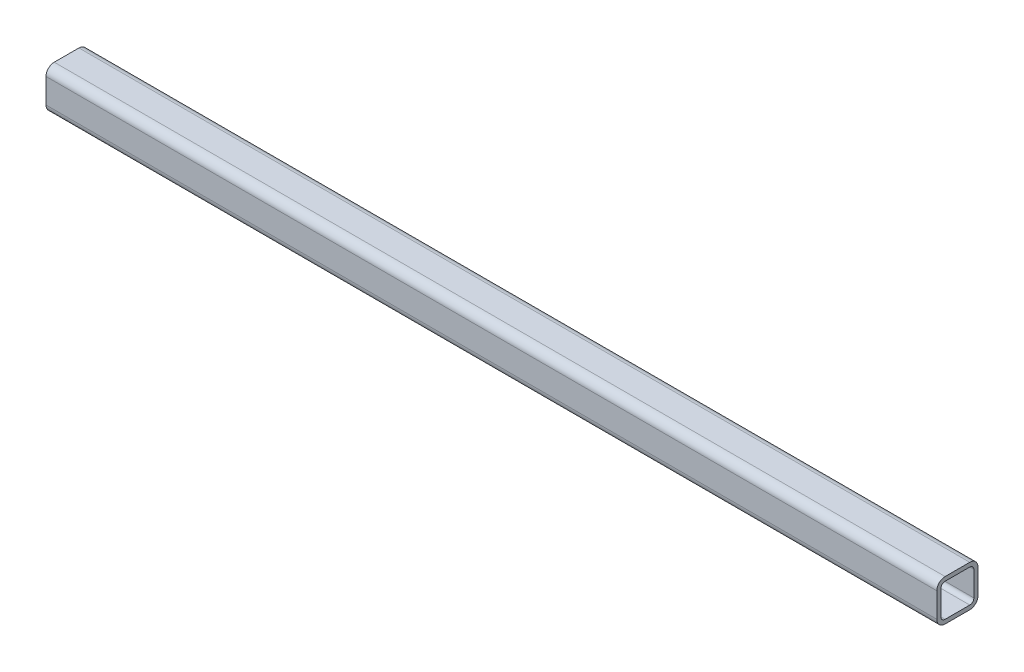
from build123d import *

# Parameters (mm, degrees)
GB_6728_1986_040_X_40_X_4_1_DEPTH = 866


with BuildPart() as part:
    # Sketch1 → Gb／6728-1986方形空心型钢 040 X 40 X 4(1) (new body)
    with BuildSketch(Plane(origin=(-433, 0, 0), x_dir=(0, 0, -1), z_dir=(1, 0, 0))):
        with BuildLine():
            Line((-12, -20), (12, -20))
            ThreePointArc((12, -20), (17.656854249, -17.656854249), (20, -12))
            Line((20, -12), (20, 12))
            ThreePointArc((20, 12), (17.656854249, 17.656854249), (12, 20))
            Line((12, 20), (-12, 20))
            ThreePointArc((-12, 20), (-17.656854249, 17.656854249), (-20, 12))
            Line((-20, 12), (-20, -12))
            ThreePointArc((-20, -12), (-17.656854249, -17.656854249), (-12, -20))
        make_face()
        with BuildLine():
            Line((-12, -16), (12, -16))
            ThreePointArc((12, -16), (14.828427125, -14.828427125), (16, -12))
            Line((16, -12), (16, 12))
            ThreePointArc((16, 12), (14.828427125, 14.828427125), (12, 16))
            Line((12, 16), (-12, 16))
            ThreePointArc((-12, 16), (-14.828427125, 14.828427125), (-16, 12))
            Line((-16, 12), (-16, -12))
            ThreePointArc((-16, -12), (-14.828427125, -14.828427125), (-12, -16))
        make_face(mode=Mode.SUBTRACT)
    extrude(amount=GB_6728_1986_040_X_40_X_4_1_DEPTH)


solid = part.part
